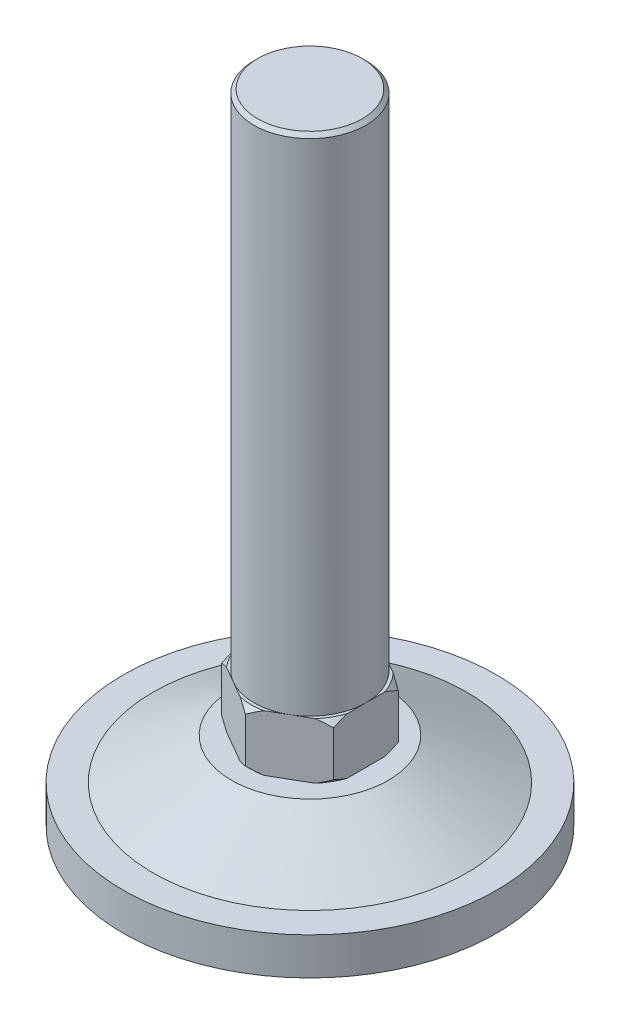
SolidWorks part; units mm, degrees
material "普通碳钢"
ref_plane "Front Plane" through (0, 0, 0) normal (0, 0, 1) x (1, 0, 0)
ref_plane "Top Plane" through (0, 0, 0) normal (0, 1, 0) x (1, 0, 0)
ref_plane "Right Plane" through (0, 0, 0) normal (1, 0, 0) x (0, 0, -1)
sketch "Sketch1" plane through (0, 0, 0) normal (0, 0, 1) x (1, 0, 0)
  line L0 (35, 0) -> (60, 0)
  line L1 (60, 0) -> (60, 9.5)
  line L2 (60, 20) -> (42, 20)
  line L3 (42, 20) -> (21, 31)
  line L4 (21, 31) -> (15, 31)
  line L5 (15, 31) -> (15, 181)
  line L6 (15, 181) -> (0, 181)
  line L7 (0, 181) -> (0, 15)
  line L8 (60, 10) -> (59.189, 10) construction
  line L9 (60, 10.5) -> (59.5, 10)
  line L10 (59.5, 10) -> (60, 9.5)
  line L11 (0, 15) -> (14, 15)
  line L12 (14, 15) -> (35, 0)
  line L13 (55, 0) -> (-55, 0) construction
  line L14 (60, 10.5) -> (60, 20)
  line L15 (0, 15) -> (0, 0) construction
  point P0 (7.5, 181)
  dimension "D1" = 20
  dimension "D2" = 181
  dimension "D3" = 15
  dimension "D4" = 6
  dimension "D5" = 31
  dimension "D6" = 18
  dimension "D7" = 60
  dimension "D8" = 10
  dimension "D9" = 0.5
  dimension "D10" = 1
  dimension "D11" = 0.5
  dimension "D12" = 15
  dimension "D13" = 25
  dimension "D14" = 14
  dimension "D15" = 45
revolve "Revolve1" add sketch "Sketch1" angle 360 about L7
cosmetic thread "Cosmetic Thread1" parameters "D2"=29
cosmetic thread "Cosmetic Thread2" parameters "D2"=29
sketch "Sketch2" plane through (0, 31, 0) normal (0, 1, 0) x (1, 0, 0)
  line L1 (15, 8.6603) -> (0, 17.3205)
  line L2 (0, 17.3205) -> (-15, 8.6603)
  line L3 (-15, 8.6603) -> (-15, -8.6603)
  line L4 (-15, -8.6603) -> (0, -17.3205)
  line L5 (0, -17.3205) -> (15, -8.6603)
  line L6 (15, -8.6603) -> (15, 8.6603)
  circle A0 centre (0, 0) radius 15 construction
  dimension "D1" = 30
extrude "Boss-Extrude1" add sketch "Sketch2" along normal blind 15
sketch "Sketch3" plane through (0, 0, 0) normal (1, 0, 0) x (0, 0, -1)
  line L0 (15.8205, 31) -> (17.3205, 32.5)
  line L1 (8.6603, 31) -> (17.3205, 31) construction
  line L2 (17.3205, 46) -> (17.3205, 31) construction
  line L3 (17.3205, 32.5) -> (17.3205, 31)
  line L4 (17.3205, 44.5) -> (15.8205, 46)
  line L5 (8.6603, 46) -> (12.9904, 46) construction
  line L6 (15.8205, 46) -> (17.3205, 46)
  line L7 (17.3205, 46) -> (17.3205, 44.5)
  line L8 (21, 31) -> (-21, 31) construction
  line L9 (17.3205, 31) -> (15.8205, 31)
  dimension "D1" = 45
  dimension "D2" = 1.5
  dimension "D3" = 45
  dimension "D4" = 1.5
revolve "Cut-Revolve1" cut sketch "Sketch3" angle 360 about axis through (0, 181, 0) along (0, 1, 0)
ref_plane "Plane1" through (0, 47, 0) normal (0, 1, 0) x (-1, 0, 0)
chamfer "Chamfer1" distance 1 angle 45 1 edges at (-15, 181, 0)
sketch "Sketch4" plane through (0, 20, 0) normal (0, 1, 0) x (1, 0, 0)
  circle A0 centre (0, 0) radius 50
  circle A1 centre (0, 0) radius 79.8617
  dimension "D1" = 100
extrude "Cut-Extrude1" cut sketch "Sketch4" against normal through all
sketch "Sketch5" plane through (0, 0, 0) normal (0, 0, 1) x (1, 0, 0)
  line L0 (50, 20) -> (-50, 20) construction
  line L1 (-57.5772, 10) -> (94.1324, 10)
  line L2 (-57.5772, 10) -> (-57.5772, -23.0316)
  line L3 (-57.5772, -23.0316) -> (94.1324, -23.0316)
  line L4 (94.1324, 10) -> (94.1324, -23.0316)
  dimension "D1" = 10
extrude "Cut-Extrude2" cut sketch "Sketch5" against normal through all both and the other way through all
